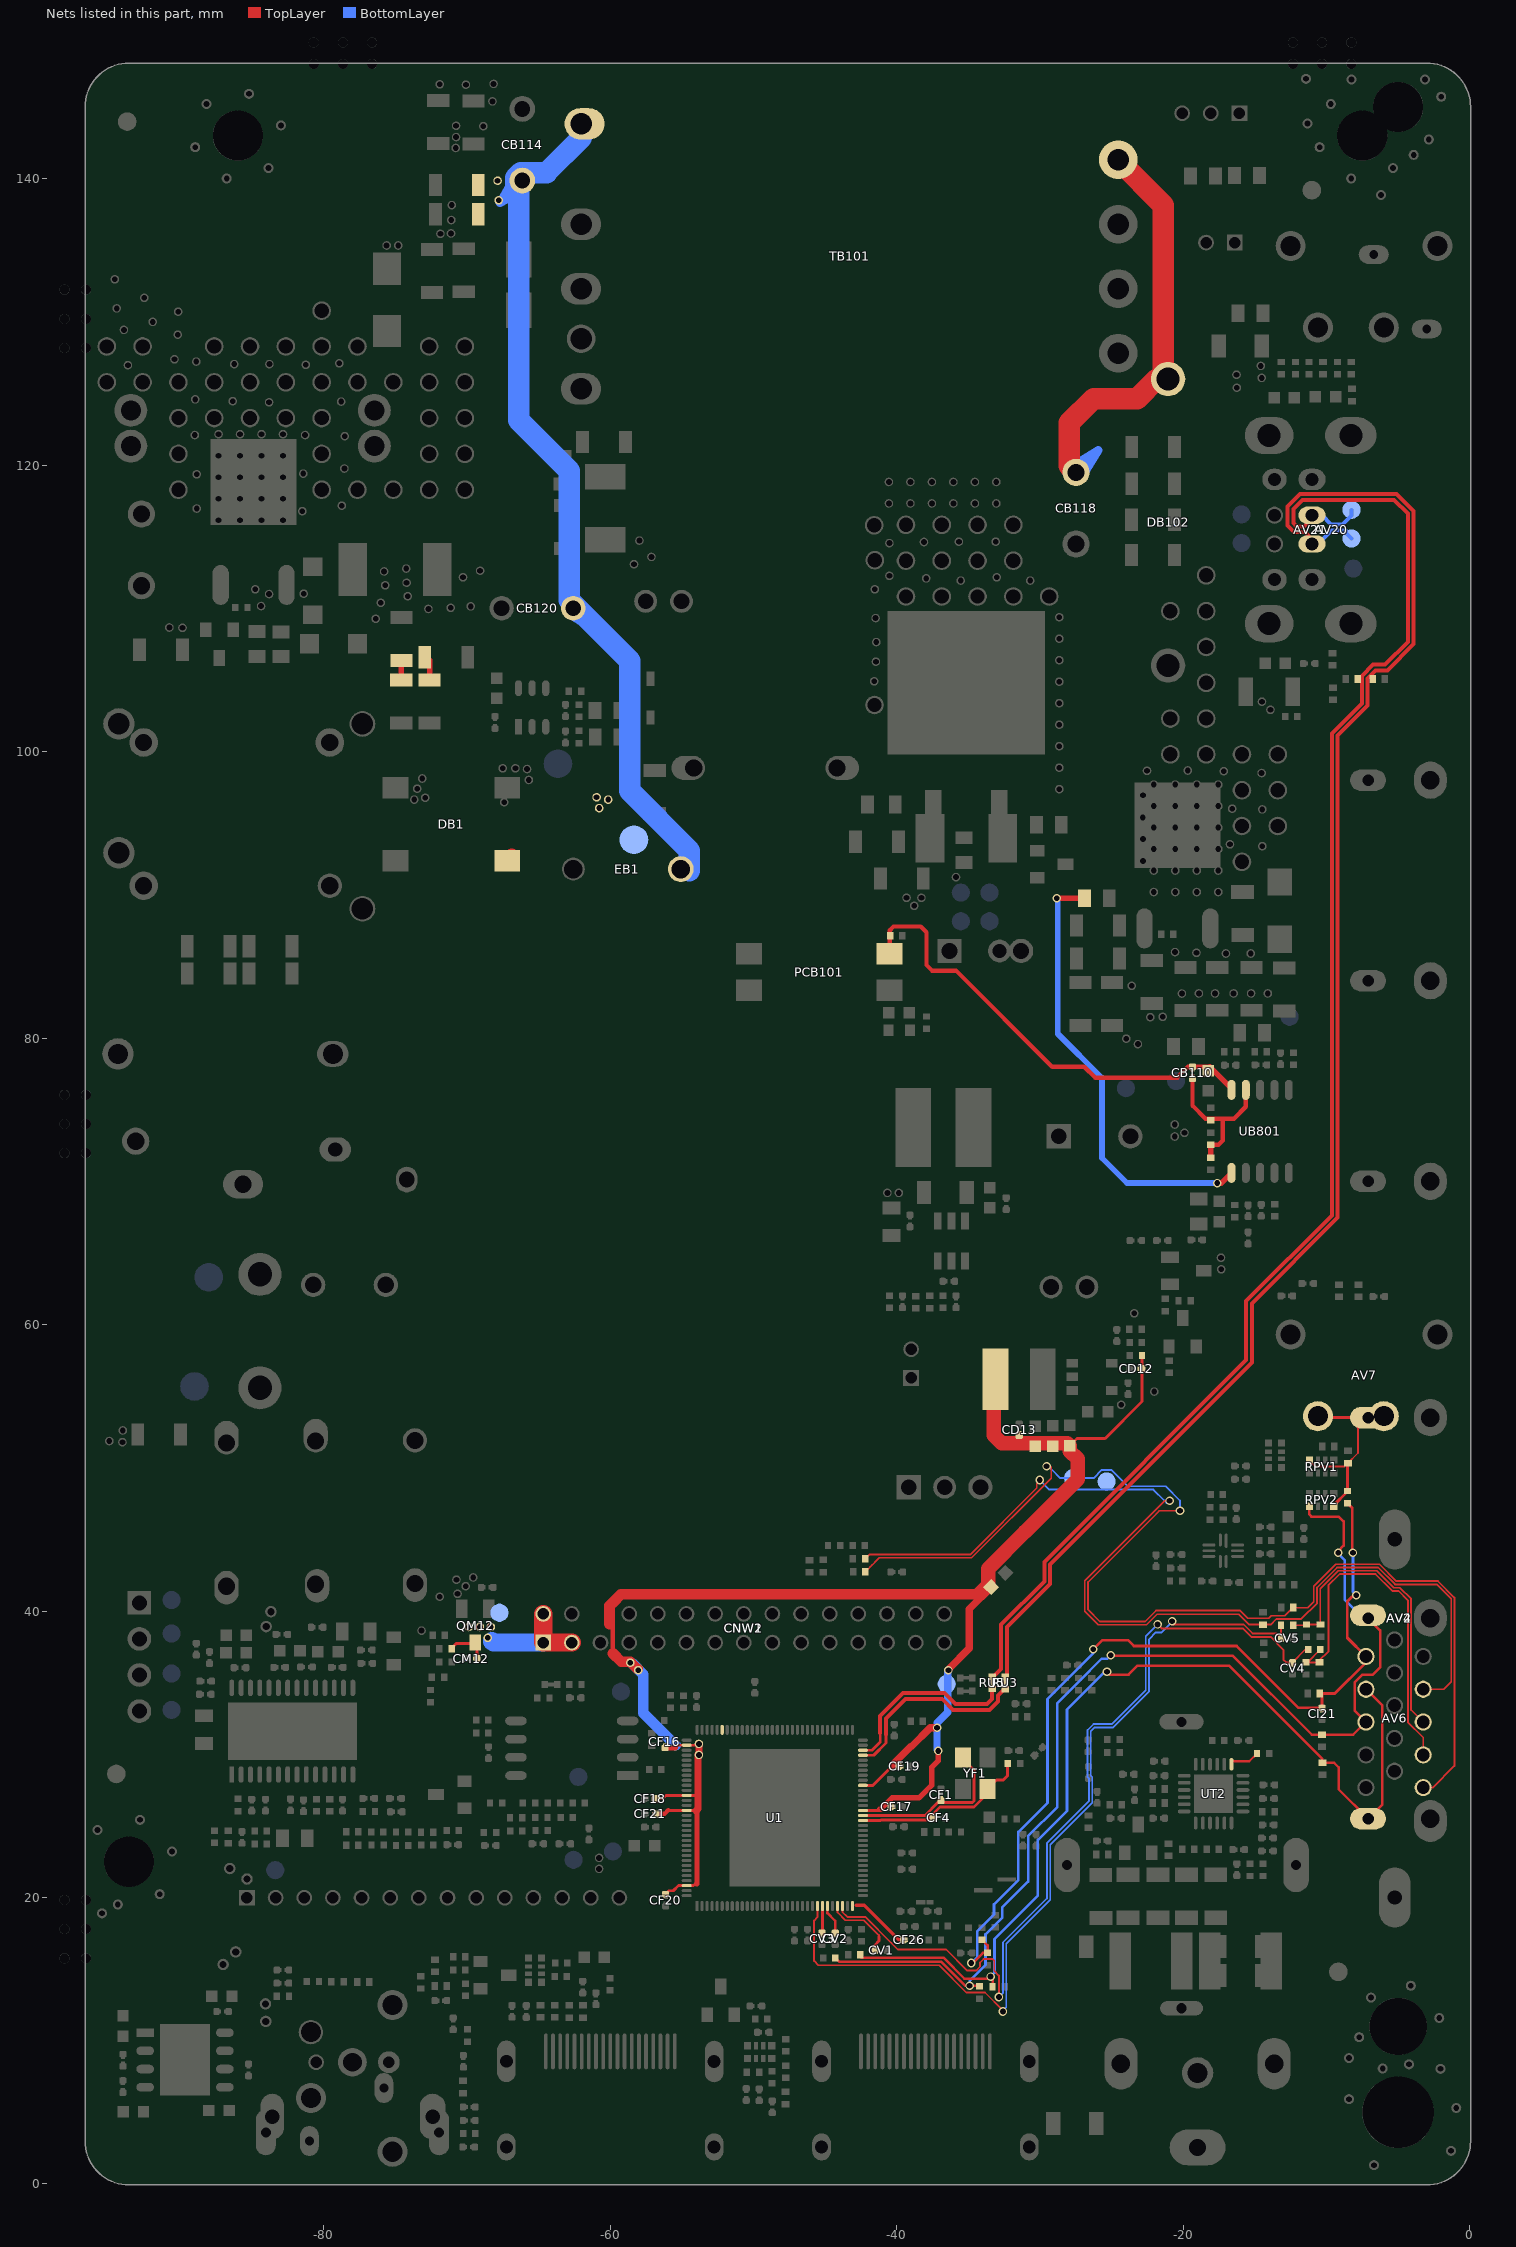
[diagram p0: the nets of this part, all layers, seen from the top]
# Altium PCB MISC86372.PcbDoc (part 14 of 16)
Units mm, origin at the board's own origin, x right, y up, seen from the top; angles counter-clockwise.
Board outline 96.73 x 148.13 mm, 2 copper layers (TopLayer, BottomLayer), stack 1.571 mm thick; 578 components, 318 nets, 2702 pads, 836 vias.

## Via types
v1: diameter 0.6, hole 0.4, TopLayer to BottomLayer, tented both sides, 816 vias
v2: diameter 0.7, hole 0.5, TopLayer to BottomLayer, tented both sides, 15 vias
v3: diameter 0.8, hole 0.5, TopLayer to BottomLayer, tented both sides, 5 vias

## Nets (pads, with @x,y where several pads share a name; then routed paths per layer and width w, separated by ;. In a path a pad name is that pad's centre, name@x,y a point inside that pad or via, vN(x,y) a via of type N, cw(c..) or ccw(c..) an arc to the next point about the centre after c; other vN are vias at no path point) (continued)
USB1_DM_IO: AV20.2@-11.01,114.5 AV21.6 DM1.1 DU1.K RU3.2 RU3.3 | length 110.6
  TopLayer w0.279: RU3.2@-32.41,35.401 -32.309,35.502 -32.309,38.88 -29.287,41.902 -29.287,43.262 -15.207,57.343 -15.207,61.472 -9.22,67.459 -9.22,101.109 -7.127,103.202 -7.127,105.106 -6.569,105.664 -5.743,105.664 -3.912,107.496 -3.912,116.78 -5.115,117.983 -11.852,117.983 -12.725,117.11 -12.725,115.783 -12.259,115.316 -11.506,115.316 -11.01,114.82 AV21.6@-11.01,114.5
  BottomLayer w0.279: AV21.6@-11.01,114.5 -10.595,114.5 -9.652,115.443 -8.636,115.443 -8.636,115.262 DM1.1@-8.251,114.876
USB1_DM_IO_IC: RU3.1 U1.61 | length 13.7
  TopLayer w0.203: U1.61@-42.362,29.931 -41.61,29.931 -40.748,30.793 -40.748,31.369
  TopLayer w0.279: -40.748,31.369 -40.748,31.409 -40.738,31.42 ; -40.748,31.431 -40.748,32.508 -39.399,33.858 -36.825,33.858 -36.063,33.096 -33.517,33.096 -32.928,33.685 -32.928,34.107 -32.536,34.499 RU3.1@-32.41,34.499
USB1_DP_IO: AV20.3 AV21.7 DP1.1 DU2.K RU5.2 RU5.3 | length 108.9
  TopLayer w0.279: RU5.2@-33.335,35.415 -33.261,35.415 -32.715,35.961 -32.715,39.049 -29.693,42.07 -29.693,43.431 -15.613,57.511 -15.613,61.64 -9.627,67.627 -9.627,101.277 -7.534,103.37 -7.534,105.275 -6.738,106.07 -5.912,106.07 -4.318,107.664 -4.318,116.611 -5.284,117.577 -11.684,117.577 -12.319,116.942 -12.319,115.951 -12.09,115.722 -11.582,115.722 -11.01,116.295 AV21.7@-11.01,116.5
  BottomLayer w0.279: AV21.7@-11.01,116.5 -10.328,116.5 -9.677,115.849 -8.89,115.849 -8.251,116.489 DP1.1@-8.251,116.876
USB1_DP_IO_IC: RU5.1 U1.62 | length 12.9
  TopLayer w0.203: U1.62@-42.362,30.281 -41.727,30.281 -41.155,30.853 -41.155,31.496
  TopLayer w0.279: -41.155,31.496 -41.155,32.676 -39.567,34.264 -36.656,34.264 -35.895,33.503 -33.685,33.503 -33.335,33.853 -33.335,34.501 RU5.1@-33.323,34.513
VBL-COIL: CB118.1 DB102.A TB101.10 | length 28.6
  TopLayer w1.5: CB118.1@-27.483,119.492 -27.956,119.966 -27.956,122.945 -26.264,124.638 -23.216,124.638 -21.844,126.009 DB102.A@-21.057,126.009 -21.387,126.34 -21.387,138.151 -24.538,141.302 TB101.10@-24.538,141.319
VBL_CTRL: U1.91
Vbridge: CB114.1@-66.142,139.865 CB120.2 DB1.1 EB1.1 pad.VIA5@-60.147,96.647 pad.VIA5@-60.776,96.054 pad.VIA5@-60.955,96.809 pad.VIA5@-67.793,138.481 pad.VIA5@-67.869,139.852 RB152.2 RB153.2 TB101.1 TP-TDT.1 | length 61.2
  TopLayer w1.016: DB1.1@-66.89,92.167 DB1.1@-66.89,92.725
  TopLayer w1.5: TB101.1@-62.085,143.866 TB101.1@-62.038,143.819
  BottomLayer w1.5: TB101.1@-62.038,143.819 -62.038,142.838 -64.451,140.426 -66.243,140.426 -66.599,140.07 -66.599,139.687 -66.599,139.563 -66.397,139.361 -66.396,139.36 -66.396,123.125 -62.865,119.594 -62.865,110.566 -61.495,109.197 -58.649,106.35 -58.649,97.257 -54.483,93.091 -54.483,91.694 EB1.1@-54.852,92.037
VBRO: RB141.1 RB142.2 | length 1.8
  TopLayer w0.381: RB142.2@-72.899,106.655 -72.619,106.374 RB141.1@-72.619,105.005
VCC_PANEL: CM12.1 CNW1.1 CNW1.2 CNW1.3 CNW2.1 CNW2.2 CNW2.3 pad.VIA5@-68.34,38.887 pad.VIA5@-68.555,38.125 pad.VIA5@-69.108,38.887 pad.VIA5@-69.875,38.887 QM12.D RM15.1 VCC_PANEL.1 | length 10.6
  TopLayer w0.203: RM15.1@-71.076,37.363 -71.076,37.404 -70.736,37.744 QM12.D@-69.317,37.744 ; QM12.D@-69.484,37.744 QM12.D@-69.422,37.807 ; CM12.1@-69.294,36.68 QM12.D@-69.294,37.679
  TopLayer w1.27: CNW2.2@-64.681,39.796 CNW2.1@-64.681,37.796 CNW2.3@-62.681,37.796
  BottomLayer w1.27: -68.25,37.887 -68.159,37.796 CNW2.1@-64.681,37.796
VCOM0: CF26.1 U1.32 | length 4.4
  TopLayer w0.254: -42.824,19.456 -42.273,19.456 -39.86,17.043 CF26.1@-39.414,17.043
VCOMP: CB109.1 CB110.1 PCB101.2 RB132.1 UB801.10 | length 32.8
  TopLayer w0.3: PCB101.2@-40.515,85.877 -40.481,85.912 -40.481,87.529 -40.227,87.782 -38.319,87.782 -37.926,87.389 -37.926,85.094 -37.541,84.709 -35.865,84.709 -29.154,77.999 -26.91,77.999 -26.148,77.237 -20.426,77.237 -19.666,77.997 CB110.1@-19.355,77.997 ; CB110.1@-19.355,77.999 CB109.1@-18.163,77.999
  TopLayer w0.381: PCB101.2@-40.515,85.877 PCB101.2@-40.107,85.877 ; CB109.1@-18.163,77.999 -16.643,76.479 UB801.10@-16.643,76.382
VDDC_CORE: CD10.2 CD12.2@-22.873,56.911 CD12.2@-23.048,56.911 CD13.2@-31.453,52.229 CD13.2@-31.453,52.404 CD14.2 CD15.2 CF15.2 CF16.2@-56.185,30.436 CF16.2@-56.185,30.611 CF17.2@-40.43,26.34 CF17.2@-40.255,26.34 CF18.1 CF19.1 CF20.2@-56.138,20.063 CF20.2@-56.138,20.238 CF21.1 LD2.1 pad.VIA5@-53.811,29.954 pad.VIA5@-53.811,30.722 pad.VIA5@-58.054,35.871 pad.VIA5@-58.602,36.394 RD9.1 U1.50 U1.55 U1.98 U1.108 U1.111 U1.126 VDDC_CORE.1 | length 121.2
  TopLayer w0.203: CF18.1@-56.784,26.898 -56.348,26.898 -56.114,27.131 -53.882,27.131 ; CF20.2@-56.138,20.238 -55.903,20.472 -55.604,20.472 -55.246,20.831 -54.18,20.831 -53.946,21.065 ; -55.964,26.088 -55.957,26.081 -53.984,26.081 -53.946,26.081 ; -55.474,30.505 -55.348,30.631 U1.98@-54.664,30.631 ; -55.333,30.631 U1.98@-54.664,30.631 ; pad.VIA5@-53.916,30.631 U1.98@-54.664,30.631 ; U1.50@-42.362,26.081 -41.262,26.081 ; U1.55@-42.362,27.831 -41.649,27.831 -40.344,29.136 ; CD10.2@-27.911,51.541 -27.408,52.045 -25.45,52.045 -22.872,54.622 RD9.1@-22.872,57.625
  TopLayer w0.305: -59.816,37.024 -59.816,40.598 -59.816,40.792 ; CF21.1@-56.792,25.835 -56.217,25.835 -55.964,26.088
  TopLayer w0.381: CF16.2@-56.134,30.436 -55.474,30.436 ; -53.974,20.975 -53.946,21.004 -53.946,21.065 -53.946,26.081 ; -41.193,26.15 -41.122,26.15 -40.322,26.949 -38.45,26.949 -37.549,27.851 -37.549,29.103 -37.113,29.539 v1(-37.113,30.235) ; CF19.1@-39.894,29.136 CF19.1@-39.871,29.159
  TopLayer w0.508: -53.984,26 -53.984,26.081 -53.984,26.09 -53.882,26.191 -53.882,27.131 pad.VIA5@-53.882,30.01 ; pad.VIA5@-53.882,29.883 pad.VIA5@-53.811,29.954 pad.VIA5@-53.811,30.722 pad.VIA5@-53.811,30.726 ; -40.234,29.159 -40.234,29.339 ; -40.143,29.431 -39.027,30.547 -38.967,30.547 -37.662,31.852 v1(-37.186,31.852) ; v1@-36.394,35.937 -34.938,37.393 -34.938,40.145 -33.912,41.171
  TopLayer w0.762: -60.044,39.107 -60.044,40.37 -59.816,40.598 -59.243,41.171 -36.297,41.171 ; -59.816,37.024 -59.801,37.024 -59.235,36.459 -58.604,36.459 pad.VIA5@-58.114,35.968 ; -35.856,41.171 -36.297,41.171 ; -34.239,41.171 -36.297,41.171
  TopLayer w1.016: -34.239,41.171 -33.62,41.79 -33.62,42.954 -31.048,45.525 ; LD2.1@-33.243,56.22 -33.243,52.285 -32.685,51.726 -28.096,51.726 CD10.2@-27.911,51.541 -27.91,51.54 -27.91,51.16 -27.377,50.627 -27.377,49.196 -31.006,45.568
  BottomLayer w0.508: v1@-37.186,30.307 v1(-37.186,31.852) -37.186,32.182 ; -37.176,32.192 -36.443,32.925 v1@-36.443,35.823
  BottomLayer w0.762: pad.VIA5@-58.427,36.306 -57.696,35.576 -57.696,32.88 -55.447,30.631
  other v1: -36.394,35.872
VGA_HS_IN: AV6.13 DV7.K RV8.2 RV9.1 | length 21
  TopLayer w0.127: RV9.1@-12.326,39.012 -11.442,39.012 RV8.2@-11.396,39.058 DV7.K@-10.431,39.058 -10.431,41.547 -9.166,42.812 -6.49,42.812 -5.309,41.631 -4.877,41.631 -4.089,40.843 -4.089,33.092 AV6.13@-3.247,32.25
VGA_HS_IN_IC: CV5.2@-12.989,38.093 CV5.2@-13.164,38.093 RV9.2 U1.25 | length 61
  TopLayer w0.127: U1.25@-45.538,19.406 -45.538,18.616 -45.771,18.383 -45.771,15.57 -45.466,15.265 -37.04,15.265 -35.143,13.368 -33.841,13.368 -32.588,12.116 v1(-32.588,12.04) ; v1(-20.777,39.294) -20.825,39.246 -20.825,39.065 -15.795,39.065 -15.166,38.436 -13.508,38.436 CV5.2@-13.176,38.104 ; RV9.2@-13.176,39.012 CV5.2@-13.176,38.104 ; CV5.2@-13.164,38.093 CV5.2@-13.176,38.104
  BottomLayer w0.127: v1@-32.588,12.116 -32.36,12.344 -32.36,16.764 -29.286,19.837 -29.286,23.694 -26.357,26.623 -26.357,28.415 -26.456,28.513 -26.456,31.594 -26.173,31.877 -24.892,31.877 -22.384,34.385 -22.384,38.03 -21.907,38.506 -21.514,38.506 -20.777,39.243 v1(-20.777,39.294)
VGA_SCL&UART_RX: AV6.15 DV1.K RF11.2 UART_RX.1 | length 83.7
  TopLayer w0.127: RF11.2@-42.196,42.739 -41.863,43.072 ; -41.706,43.229 -41.863,43.072 ; v1(-29.54,50.114) -29.294,50.114 -29.218,50.038 -29.218,49.277 -34.782,43.713 -41.222,43.713 -41.863,43.072 ; -21.724,46.947 -21.868,46.802 ; v1(-20.225,47.001) -21.67,47.001 -21.868,46.802 ; DV1.K@-12.377,40.208 DV1.K@-12.351,40.234 ; DV1.K@-12.349,40.275 -12.351,40.273 DV1.K@-12.351,40.234 ; DV1.K@-12.308,40.234 -11.296,40.234 -10.888,40.642 -10.888,41.736 -9.355,43.269 -6.301,43.269 -5.119,42.088 -2.217,42.088 -1.067,40.938 -1.067,29.185 -2.581,27.67 AV6.15@-3.247,27.67 ; -21.868,46.802 -26.645,42.026 -26.645,40.088 -25.826,39.27 -22.662,39.27 -21.901,40.03 -16.021,40.03 -15.491,39.5 -14.043,39.5 -13.868,39.675 -12.91,39.675 DV1.K@-12.351,40.234
  BottomLayer w0.127: v1(-29.54,50.114) -29.42,50.114 -29.023,49.717 ; -28.759,49.453 -29.023,49.717 ; v1(-20.225,47.001) -20.225,47.708 -21.222,48.704 -23.875,48.704 -25.018,49.847 -25.681,49.847 -26.252,49.276 UART_RX.1@-27.686,49.276 -28.582,49.276 -29.023,49.717
VGA_SDA&UART_TX: AV6.12 DV2.K RF10.2 UART_TX.1 | length 73.1
  TopLayer w0.127: RF10.2@-42.214,43.649 -41.921,43.942 -34.876,43.942 -30.23,48.588 -30.23,48.878 -29.832,49.276 -29.896,49.276 v1(-30.023,49.149) ; v1(-20.955,47.701) -21.293,47.701 -26.873,42.121 -26.873,39.993 -25.921,39.041 -22.567,39.041 -21.832,39.776 -16.126,39.776 -15.403,39.053 DV2.K@-14.427,39.053 -13.88,39.053 -13.487,39.446 -11.76,39.446 -10.659,40.547 -10.659,41.642 -9.26,43.04 -6.395,43.04 -5.214,41.859 -2.311,41.859 -1.295,40.843 -1.295,35.052 -1.807,34.54 AV6.12@-3.247,34.54
  BottomLayer w0.127: v1(-30.023,49.149) -29.35,48.476 -22.085,48.476 -21.324,47.714 ; v1@-21.158,47.549 -21.324,47.714 ; v1(-20.955,47.701) -20.968,47.714 -21.324,47.714 ; AV6.12@-3.247,34.54 AV6.12@-3.236,34.551
VGA_VS_IN: AV6.14 DV6.K RV6.2 RV7.1 | length 25.6
  TopLayer w0.127: RV7.1@-10.421,37.313 -11.317,36.417 DV6.K@-10.49,36.417 -10.49,36.548 -9.868,37.17 -9.868,41.786 -9.071,42.583 -6.585,42.583 -5.404,41.402 -4.972,41.402 -4.318,40.748 -4.318,32.239 -3.247,31.168 AV6.14@-3.247,29.96
VGA_VS_IN_IC: CV4.2@-12.37,36.242 CV4.2@-12.37,36.417 RV7.2 U1.30 | length 59.9
  TopLayer w0.127: U1.30@-43.788,19.406 -43.788,18.977 -43.455,18.644 -42.196,18.644 -40.376,16.824 -39.921,16.369 -36.547,16.369 -35.073,14.894 -34.458,14.894 -34.188,15.164 -34.188,15.455 -33.946,15.697 -33.299,15.697 -33.198,15.596 -33.198,14.882 -32.868,14.552 v1@-32.868,13.081 ; v1@-32.842,13.056 v1@-32.868,13.081 ; v1(-21.793,39.065) -21.511,38.783 -15.836,38.783 -15.243,38.19 -13.904,38.19 -13.005,37.291 -13.005,36.6 -12.821,36.417 CV4.2@-12.37,36.417 CV4.2@-12.363,36.424 ; CV4.2@-12.37,36.424 CV4.2@-12.363,36.424 ; CV4.2@-12.344,36.424 CV4.2@-12.363,36.424 ; RV7.2@-11.271,37.313 -11.474,37.313 CV4.2@-12.363,36.424 ; v1@-32.868,13.081 -32.893,13.106 -32.893,13.081 v1(-32.868,13.056) v1@-32.868,13.081
  BottomLayer w0.127: v1@-32.842,13.056 -32.588,13.31 -32.588,16.859 -29.515,19.932 -29.515,23.788 -26.586,26.717 -26.586,28.32 -26.684,28.418 -26.684,31.689 -26.267,32.106 -24.987,32.106 -22.612,34.48 -22.612,38.246 v1(-21.793,39.065)
VGS1: RB807.1 UB801.1 | length 31.4
  TopLayer w0.4: v1(-28.829,89.764) RB807.1@-26.899,89.764 ; v1(-17.628,69.875) -17.337,69.875 UB801.1@-16.63,70.582
  BottomLayer w0.4: v1(-28.829,89.764) -28.766,89.7 -28.766,80.302 -25.679,77.216 -25.679,71.628 -23.927,69.875 v1(-17.628,69.875)
VREF: CB110.2@-19.355,77.147 CB110.2@-19.355,77.322 RB133.1 RB134.2 RB135.2 UB801.9 | length 11.1
  TopLayer w0.3: CB110.2@-19.355,77.322 -19.355,75.284 -18.442,74.371 -17.247,74.371 ; RB134.2@-18.085,72.549 -17.545,72.549 -17.247,72.847 -17.247,74.371 ; UB801.9@-15.63,76.382 -15.63,75.2 -16.459,74.371 -17.247,74.371
  TopLayer w0.381: RB135.2@-18.085,71.647 RB134.2@-18.085,72.549
VSTB: RB101.2 RB102.2 | length 2
  TopLayer w0.381: RB101.2@-74.6,105.005 -74.6,106.323 RB102.2@-74.574,106.348 -74.574,105.671
XTAL_IN_IC: CF4.2@-37.309,25.552 CF4.2@-37.484,25.552 RF24.2 U1.48 YF1.3 | length 12.4
  TopLayer w0.203: U1.48@-42.363,25.381 -41.132,25.381 -41.113,25.4 -37.901,25.4 -36.987,26.314 -34.617,26.314 -33.493,27.439 -33.493,27.752 -33.046,28.199 -32.563,28.199 -32.264,28.498 RF24.2@-32.264,29.362
XTAL_OUT: L6.2 UT2.13 | length 2.1
  TopLayer w0.152: UT2.13@-16.637,29.637 -16.51,29.51 -15.384,29.51 L6.2@-14.852,30.041
XTAL_OUT_IC: CF1.2@-36.906,26.753 CF1.2@-36.906,26.928 U1.49 YF1.1 | length 11.5
  TopLayer w0.203: U1.49@-42.362,25.731 -38.038,25.731 -37.149,26.619 -34.743,26.619 -34.615,26.747 -34.615,28.9 -35.369,29.654 YF1.1@-35.369,29.777
YPP_Pb&B_IN&AU_L: AV2.3 AV4.3 AV6.3 DV5.K RPV2.1 RV5.2 RV10.1 | length 78.2
  TopLayer w0.18: RV10.1@-44.279,15.773 -44.026,15.521 -36.898,15.521 v1@-35.214,13.836 ; v1(-34.916,13.836) -34.257,13.836 RV5.2@-34.214,13.793 ; v1@-25.051,36.887 -16.55,36.887 -11.025,31.362 DV5.K@-10.312,31.362 -8.135,31.362 AV6.3@-7.247,32.25 -8.039,33.042 -8.039,34.996 -7.475,35.56 -6.756,35.56 -6.253,36.063 -6.253,38.653 AV2.3@-7.1,39.5 ; RPV2.1@-11.192,47.309 -11.192,46.742 -11.045,46.595 -9.145,46.595 -8.802,46.252 -8.802,44.567 -9.169,44.2 v1(-9.169,44.069)
  BottomLayer w0.18: v1@-34.916,14.074 -34.916,14.177 -33.807,15.285 -33.807,17.424 -32.648,18.584 -32.648,19.287 -30.823,21.112 -30.823,23.571 -30.823,24.292 -28.79,26.326 -28.79,33.571 -27.302,35.059 -25.689,36.672 -25.304,36.672 ; v1@-9.169,43.994 -8.726,43.551 -8.726,40.818 -7.408,39.5 AV2.3@-7.1,39.5 ; AV6.3@-7.247,32.25 AV6.3@-7.247,32.486
  other v1: -25.07,36.906
YPP_Pb&B_IN_IC: CV3.2@-45.215,17.37 CV3.2@-45.215,17.545 U1.26 | length 2
  TopLayer w0.183: CV3.2@-45.215,17.37 -45.188,17.396 -45.188,18.603 U1.26@-45.188,19.406
YPP_Pr&PC_L_IN&AV_R: AV2.5 AV4.5 AV7.4 AV7.5@-10.6,53.6 DV9.K RI4.2 RPV1.7 RPV2.7 | length 13.8
  TopLayer w0.127: RPV1.7@-11.192,50.462 RPV1.7@-11.192,50.498 ; RPV1.7@-11.192,50.532 RPV1.7@-11.192,50.498 ; DV9.K@-8.534,50.299 DV9.K@-8.509,50.324 ; AV2.5@-7.8,52.8 -7.8,51.033 DV9.K@-8.509,50.324 ; RPV1.7@-11.192,50.498 -10.782,50.089 -8.744,50.089 DV9.K@-8.509,50.324
  TopLayer w0.203: AV7.5@-10.6,53.6 -10.5,53.5 AV2.5@-7.1,53.5 AV2.5@-7.8,52.8 ; RPV2.7@-9.492,47.309 -9.492,47.386 -8.534,48.343 RI4.2@-8.534,48.38 ; RI4.2@-8.56,48.355 RI4.2@-8.534,48.38 ; DV9.K@-8.534,50.299 RI4.2@-8.534,48.38
YPP_Pr&R_IN: AV6.1 CI21.1 DV3.K RI4.1 RV1.2 RV2.1 | length 62.9
  TopLayer w0.18: v1@-34.689,15.427 -33.985,16.13 RV2.1@-33.655,16.13 -33.655,16.665 RV1.2@-34.043,17.053 ; v1(-26.284,37.326) -25.662,37.948 -23.831,37.948 -23.444,37.56 -16.271,37.56 -11.952,33.242 CI21.1@-10.312,33.242
  TopLayer w0.203: DV3.K@-10.472,34.239 -9.423,34.239 -7.247,36.415 AV6.1@-7.247,36.83 -8.553,38.136 -8.553,40.659 -8.237,40.975 ; DV3.K@-10.396,34.181 -10.396,34.188 -10.312,34.105 CI21.1@-10.312,33.242 CI21.1@-10.312,33.089 ; RI4.1@-8.534,47.53 -8.204,47.2 v1@-8.204,44.018
  BottomLayer w0.18: v1(-34.791,15.427) -34.393,15.825 -34.393,17.633 -33.209,18.816 -33.209,19.519 -31.508,21.221 -31.508,24.576 -29.474,26.609 -29.474,33.855 -26.915,36.414 v1@-26.284,37.045
  BottomLayer w0.203: v1@-8.153,43.967 -8.153,41.336 v1(-7.923,41.106) ; v1(-8.153,44.069) v1@-8.103,44.018
YPP_Pr&R_IN_IC: CV1.2@-41.347,16.307 CV1.2@-41.522,16.307 U1.29 | length 5.2
  TopLayer w0.127: U1.29@-44.138,19.406 -44.138,18.962 -43.591,18.415 -42.291,18.415 -41.25,17.374 -41.25,17.272
  TopLayer w0.203: CV1.2@-41.522,16.307 -41.522,16.693 -41.238,16.978 -41.238,17.272
YPP_Y&G_IN&AV: AV2.1 AV4.1 AV6.2 DV4.K RV3.2 RV4.1 | length 68.7
  TopLayer w0.18: RV4.1@-42.491,15.803 -36.746,15.803 -35.271,14.328 v1@-33.555,14.328 ; RV3.2@-33.299,13.793 v1@-33.299,14.412 ; v1(-25.324,35.763) -25.121,35.56 -23.821,35.56 -23.2,36.181 -16.795,36.181 -10.287,29.673 DV4.K@-10.287,29.406 -9.467,29.406 -9.144,29.083 -9.144,27.544 AV2.1@-7.1,25.5 -6.096,26.504 -6.096,33.389 AV6.2@-7.247,34.54
  BottomLayer w0.18: v1(-33.452,14.478) -33.179,14.751 -33.179,17.103 -30.15,20.132 -30.15,24.013 -28.117,26.047 -28.117,33.123 v1@-25.476,35.763
YPP_Y&G_IN_IC: CV2.2@-44.298,17.37 CV2.2@-44.298,17.545 U1.27 | length 2.3
  TopLayer w0.127: -44.838,18.956 U1.27@-44.838,19.406
  TopLayer w0.18: -44.838,18.956 -44.838,18.918 -44.298,18.377 CV2.2@-44.298,17.37
pads on no net: "Conformal Coating.0" AI_V.0 AI_V.1 AI_V.2 AV1.0 AV2.0 AV4.0 AV6.0 AV6.4 AV6.9 AV6.11 AV6.30 AV6.31 AV6.32 AV6.33 AV6.34 AV6.35 AV6.36 AV6.37 AV6.38 AV6.39 AV6.40 AV6.41 AV6.42 AV6.43 AV6.44 AV7.5@-6,53.6 AV7.5@-10.6,53.6 AV7.6 AV7.7 AV20.0 AV20.1@-11.01,114.5 AV20.2@-11.01,116.5 AV21.0 AV22.2@-78,8.5 AV22.3@-71.95,3.6 AV22.3@-84.05,3.6 AV23.0 AV41.0 AV41.8 CA3.2@-85.714,24.197 CA4.2@-74.939,25.984 CA5.2@-85.033,26.448 CA6.2@-84.075,26.448 CA7.2@-82.324,26.468 CA8.2@-81.417,26.406 CA9.2@-78.689,26.448 CA10.2@-76.864,26.92 CA11.2@-74.994,26.921 CA12.2@-88.243,35.105 CA13.2@-88.268,34.188 CA14.2@-85.852,36.043 CA15.2@-83.077,36.069 CA16.2@-81.208,36.086 CA17.2@-79.063,36.068 CA18.2@-76.995,36.347 CA19.2@-77.025,37.272 CA24.2@-87.979,36.751 CA25.2@-88.9,37.338 CA26.2@-82.927,38.372 CA27.2@-80.463,38.869 CA33.2@-31.323,33.528 CB101.2@-63.129,102.87 CB103.2@-68.047,102.032 CB110.2@-19.355,77.572 CB111.2@-63.129,101.016 CB114.1@-66.142,139.865 CB114.1@-66.142,144.865 CB116.0 CB118.0 CB120.41 CB120.42 CB803.2@-15.469,67.945 CB805.2@-15.469,66.044 CB806.2@-16.713,78.105 CB812.2@-14.554,67.971 CB813.2@-13.208,78.562 CB814.2@-14.58,78.13 CD3.2@-39.079,67.231 CD4.2@-35.859,61.595 CD5.2@-39.603,61.589 CD6.2@-32.36,68.445 CD8.2@-24.638,59.233 CD9.2@-36.365,63.017 CD12.2@-23.298,56.911 CD13.2@-31.453,52.654 CD17.2@-23.849,55.525 CF1.2@-36.906,27.178 CF2.2@-68.504,30.115 CF4.2@-37.059,25.552 CF7.2@-49.911,34.671 CF8.2@-57.202,24.914 CF9.2@-40.174,31.689 CF10.2@-46.226,17.375 CF11.2@-47.14,17.375 CF12.2@-39.294,23.114 CF13.2@-39.115,17.975 CF14.2@-39.876,24.942 CF16.2@-56.185,30.861 CF17.2@-40.005,26.34 CF18.2@-57.209,26.898 CF19.2@-39.446,29.159 CF20.2@-56.138,19.813 CF21.2@-57.201,25.832 CF24.2@-40.03,28.245 CF25.2@-61.493,24.435 CF26.2@-39.116,17.043 CF27.2@-37.484,19.043 CF28.2@-39.359,19.039 CF29.2@-11.303,62.865 CF30.2@-12.769,62.001 CF31.2@-43.383,17.373 CF38.2@-31.833,30.251 CF40.2@-30.099,30.201 CG2.2@-94.027,6.802 CG4.2@-85.25,7.959 CG201.2@-40.005,42.723 CH1.2@-65.862,12.044 CH2.2@-66.861,12.049 CH3.2@-50.506,6.244 CH4.2@-61.006,12.928 CH21.2@-49.313,10.59 CH22.2@-49.828,12.421 CH81.2@-61.925,13.745 CH101.2@-48.692,5.385 CH102.2@-49.604,6.223 CI1.2@-6.35,61.951 CI2.2@-35.154,16.129 CI3.2@-16.471,41.993 CI4.2@-20.496,42.996 CI6.2@-16.007,50.126 CI8.2@-21.895,43.51 CI12.2@-16.298,46.805 CI21.2@-10.312,32.817 CI35.2@-18.335,42.088 CI36.2@-11.582,45.415 CI37.2@-14.275,45.868 CI38.2@-16.002,49.2 CI39.2@-20.502,43.94 CI41.2@-14.275,43.993 CK1.2@-62.439,33.941 CK2.2@-71,23.688 CK3.2@-63.17,23.749 CK4.2@-68.37,23.63 CK5.2@-65.056,23.752 CL4.2@-26.01,26.988 CL22.2@-94.018,8.64 CL24.2@-87.065,12.038 CM1.2@-23.306,65.863 CM2.2@-19.053,65.913 CM3.2@-21.453,65.862 CM11.2@-68.595,41.652 CM12.2@-69.694,36.68 CN1.2@-78,8.5 CN1.3@-71.95,3.6 CN1.3@-84.05,3.6 CN9.0 CN9.8 CNA1.0 CNA2.0 CNB1.109 CNB1.110 CNB2.0 CNB821.0 CNB822.0 CNB831.0 CNK1.0 CNK2.0 CNW1.0 CNW1.372 CNW1.373 CNW1.374 CNW1.375 CNW1.376 CNW1.377 CNW1.378 CNW1.379 CNW1.380 CNW1.381 CNW1.382 CNW1.383 CNW1.384 CNW1.385 CNW1.386 CNW1.387 CNW1.388 CNW1.390 CNW1.391 CNW1.392 CNW1.393 CNW1.394 CNW1.395 CNW1.396 CNW1.397 CNW1.398 CNW1.400 CNW1.401 CNW2.0 CO11.2@-70.256,8.56 CO12.2@-70.968,11.176 CO13.2@-71.831,12.802 CO14.2@-69.887,2.577 CO15.2@-69.85,4.431 CO16.2@-69.85,5.371 CO31.2@-53.975,33.681 CO32.2@-82.855,14.021 CO33.2@-82.855,14.935 CT1.2@-27.737,36.22 CT6.2@-16.259,21.95 CT7.2@-14.117,23.239 CT8.2@-26.619,28.728 CT10.2@-26.645,30.582 CT11.2@-30.277,24.003 CT12.2@-31.191,24.003 CT14.2@-25.654,23.952 CT15.2@-24.706,25.535 CT16.2@-16.129,23.343 CT17.2@-21.717,25.532 CT18.2@-23.393,27.178 CT19.2@-21.691,28.504 CT20.2@-23.829,28.6 CT21.2@-21.666,29.515 CT22.2@-14.117,24.154 CT23.2@-14.05,26.903 CT24.2@-14.072,25.07 CT25.2@-14.021,27.864 CT26.2@-39.294,21.971 CT27.2@-15.799,30.963 CU1.2@-11.197,106.147 CV1.2@-41.097,16.307 CV2.2@-44.298,17.12 CV3.2@-45.215,17.12 CV4.2@-12.37,35.992 CV5.2@-12.739,38.093 CXB1.77 CXB1.78 CYB1.61 CYB2.61 CYB3.61 CYB4.61 DB102.0 DB102.1 EA1.0 EA2.0 EA2.5 EA2.6 EB1.2@-55.076,91.796 EB1.2@-62.576,91.796 EB101.0 EB101.1@-31.323,86.081 EB101.1@-36.323,86.081 EB102.1@-32.823,86.081 EB102.1@-36.323,86.081 EB106.0 EB801.0 EB801.1@-23.687,73.139 EB801.1@-28.687,73.139 EB802.2@-28.687,73.139 EB802.3 ED1.0 ED1.5 ED1.6 FB1.4 FB1.5 GD1.0 GD2.0 GD3.0 GDT2.1@-17.502,14.554 GDT2.1@-17.502,16.586 GDT2.1@-18.501,15.52 GDT2.2@-13.503,15.52 GDT2.2@-14.501,14.554 GDT2.2@-14.501,16.586 H1.0 H2.0 H3.0 H4.0 H5.0 H6.0 JH1.0 JH21.0 LCB1.4@-79.578,90.635 LCB1.4@-79.578,100.635 LCB1.4@-92.578,90.635 LCB1.4@-92.578,100.635 LCB2.5 LCB2.6 LCB2.7 LCB2.8 M1.0 M2.0 M3.0 M4.0 Manufacture_Info.0 MOVB1.2@-85.633,69.798 MOVB1.2@-93.133,72.798 NTCB1.2@-74.208,70.121 NTCB1.3 PT1.0 RFT1.0 RFT2.0 S/N1.0 TB101.0 TB101.4 U1.0 U1.56 U1.59 UA1.13 UA1.EPAD@-79.77,30.936 UA1.EPAD@-79.77,32.286 UA1.EPAD@-81.388,30.936 UA1.EPAD@-81.388,32.286 UA1.EPAD@-83.006,30.936 UA1.EPAD@-83.006,32.286 UA1.EPAD@-84.624,30.936 UA1.EPAD@-84.624,32.286 UT2.14 UT2.21 XXXXXX.0 XXXXXXXXXXXXXX.0 用于U1.0
copper on no net: | length 86.4
  TopLayer w0.127: 167.894,51.779 167.894,53.779 ; 153.901,51.779 153.901,53.779 172.494,53.779 172.494,51.779 153.901,51.779
  BottomLayer w0.127: 167.894,46.245 167.894,48.245 ; 153.901,46.245 172.494,46.245 172.494,48.245 153.901,48.245 153.901,46.245